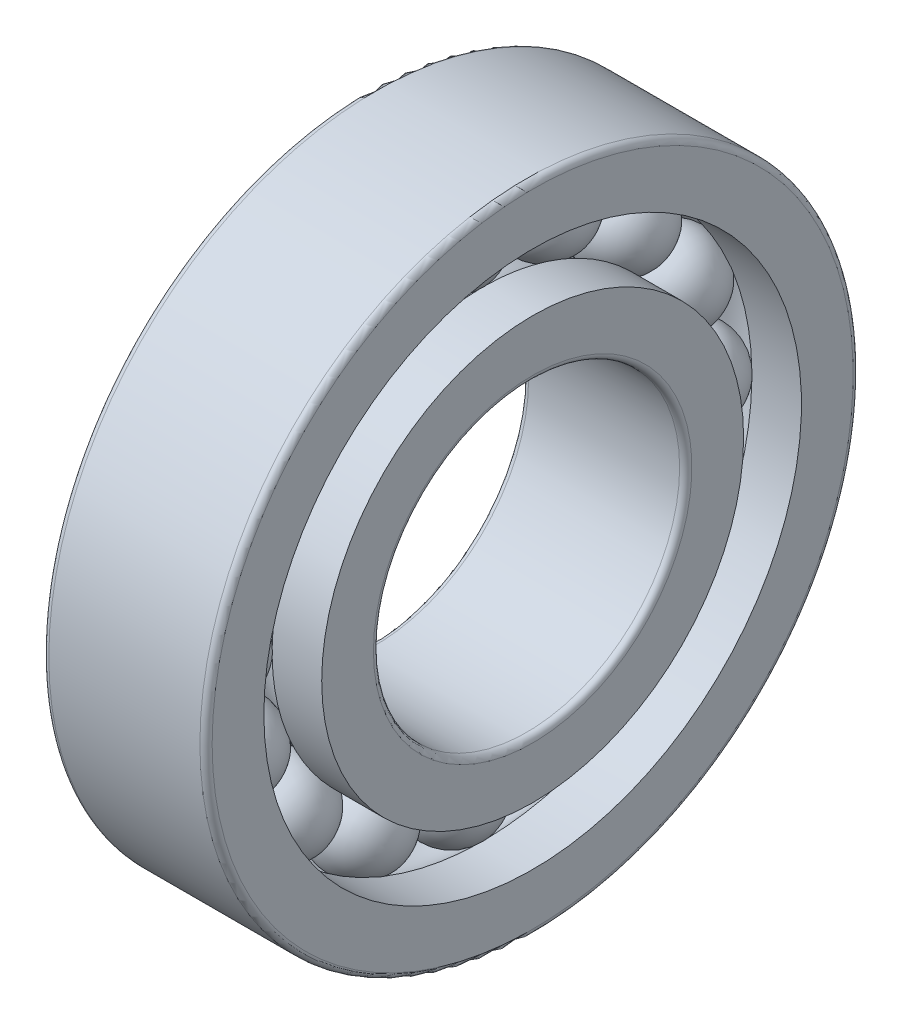
SolidWorks part; units mm, degrees
ref_plane "Front" through (0, 0, 0) normal (0, 0, 1) x (1, 0, 0)
ref_plane "Top" through (0, 0, 0) normal (0, 1, 0) x (1, 0, 0)
ref_plane "Right" through (0, 0, 0) normal (1, 0, 0) x (0, 0, -1)
sketch "Sketch1" plane through (0, 0, 0) normal (0, 0, 1) x (1, 0, 0)
  line L0 (-9.6833, 0) -> (9.8371, 0) construction
  line L1 (-2.125, 11.75) -> (2.125, 11.75)
  line L2 (-4.5966, 11.75) -> (4.6657, 11.75) construction
  arc A0 (2.125, 11.75) -> (-2.125, 11.75) centre (0, 11.75) ccw
revolve "Revolve1" add sketch "Sketch1" angle 360 about L2
sketch "Sketch2" plane through (0, 0, 0) normal (0, 0, 1) x (1, 0, 0)
  line L0 (-4, 10.3333) -> (-4, 7.5)
  line L1 (-4, 7.5) -> (4, 7.5)
  line L2 (4, 7.5) -> (4, 10.3333)
  line L3 (4, 10.3333) -> (1.5704, 10.3333)
  line L4 (-6.9714, 0) -> (8.1665, 0) construction
  line L5 (-6.7058, 11.75) -> (6.7058, 11.75) construction
  line L6 (-1.5704, 10.3333) -> (-4, 10.3333)
  arc A0 (-1.5704, 10.3333) -> (1.5704, 10.3333) centre (0, 11.75) ccw
revolve "Revolve2" add sketch "Sketch2" angle 360 about L4
sketch "Sketch3" plane through (0, 0, 0) normal (0, 0, 1) x (1, 0, 0)
  line L0 (-8.7107, 0) -> (9.1288, 0) construction
  line L1 (-4, 16) -> (4, 16)
  line L2 (-4, 16) -> (-4, 13.1667)
  line L3 (-4, 13.1667) -> (-1.5704, 13.1667)
  line L4 (4, 16) -> (4, 13.1667)
  line L5 (-7.2948, 11.75) -> (7.2948, 11.75) construction
  line L6 (1.5704, 13.1667) -> (4, 13.1667)
  arc A0 (1.5704, 13.1667) -> (-1.5704, 13.1667) centre (0, 11.75) ccw
revolve "Revolve3" add sketch "Sketch3" angle 360 about L0
pattern_circular "Circular-Pattern1" count 16 over 360 about axis through (0, 0, 0) along (1, 0, 0) of "Revolve1"
fillet "Fillet1" radius 0.3 4 edges at (-4, 0, 7.5) (-4, 0, 16) (4, 0, 16) (4, 0, 7.5)
equation "\"d0@Sketch1\" = ( \"DD@Sketch3\" + \"d@Sketch2\" )  / 2"
equation "\"dia@Sketch1\" =  ( \"DD@Sketch3\" - \"d@Sketch2\" )  / 4"
equation "\"D3@Sketch2\" = ( \"DD@Sketch3\" + \"d@Sketch2\" )  / 2 / 2"
equation "\"D4@Sketch2\" = ( \"DD@Sketch3\" - \"d@Sketch2\" )  / 6"
equation "\"D5@Sketch2\" = \"dia@Sketch1\" - 0.02"
equation "\"B/2@Sketch2\" = \"B@Sketch2\" / 2"
equation "\"D4@Sketch3\" = ( \"DD@Sketch3\" + \"d@Sketch2\" )  / 2 / 2"
equation "\"D5@Sketch3\" = ( \"DD@Sketch3\" - \"d@Sketch2\" )  / 6"
equation "\"B@Sketch3\" = \"B@Sketch2\""
equation "\"B/2@Sketch3\" = \"B@Sketch3\" / 2"
equation "\"D1@Sketch3\" = \"dia@Sketch1\" - 0.02"
equation "\"m@Circular-Pattern1\" = int( 3.14159265 / atn(( \"dia@Sketch1\" / 2) / sqr(( \"DD@Sketch3\" + \"d@Sketch2\" )  / 2 * ( \"DD@Sketch3\" + \"d@Sketch2\" )  / 2/4 - ( \"dia@Sketch1\" / 2) *  ( \"dia@Sketch1\" / 2))))-1"
